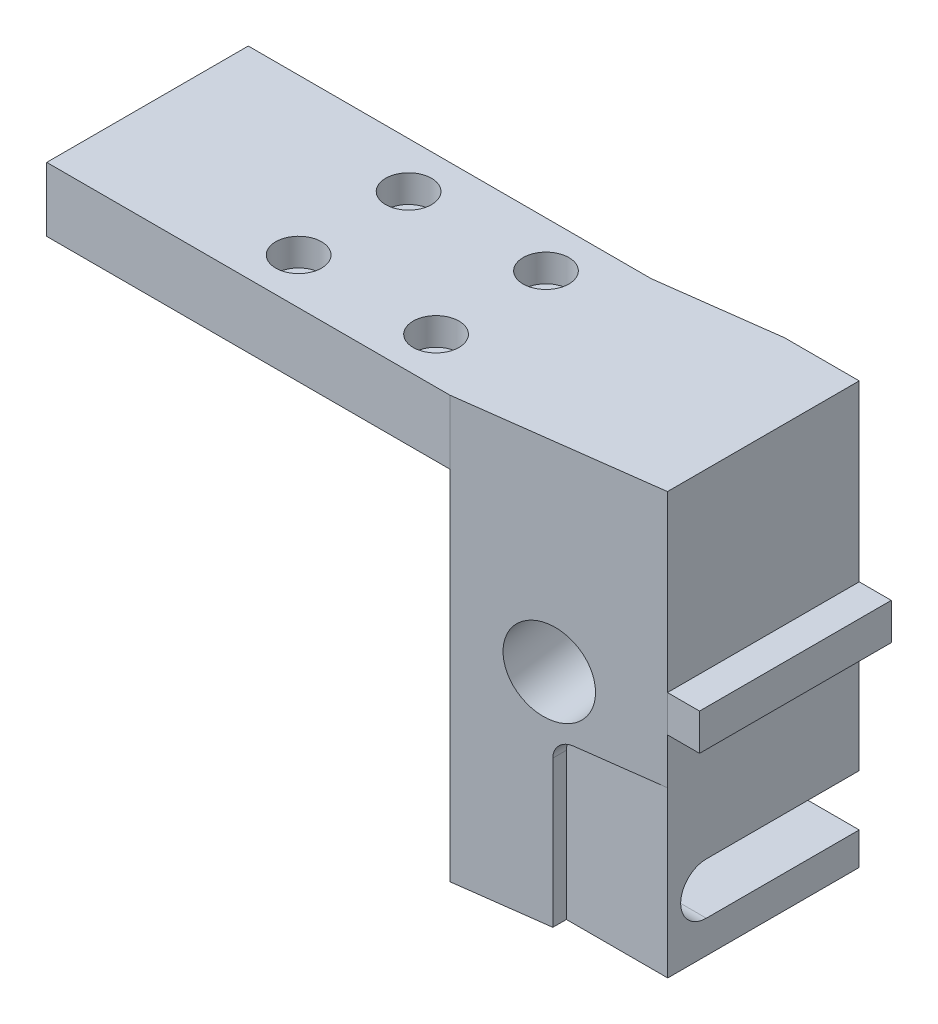
from build123d import *

# Parameters (mm, degrees)
EXTRUDE_1_DEPTH     = 23.69
CUT_EXTRUDE_1_REACH = 50.333
SKETCH_2_W          = 44
SKETCH_2_H          = 39
CUT_EXTRUDE_2_REACH = 75.348
CUT_EXTRUDE_3_DEPTH = 63.115721705
CUT_EXTRUDE_4_DEPTH = 2.79
CUT_EXTRUDE_5_REACH = 53.075
SKETCH_7_R          = 4.5
SKETCH_8_R          = 1.25
CUT_EXTRUDE_6_DEPTH = 8.5
SKETCH_10_R         = 1.45
CUT_EXTRUDE_7_DEPTH = 63.115721705
SKETCH_11_R         = 2.5
CUT_EXTRUDE_8_DEPTH = 3
SKETCH_12_R         = 2.25
CUT_EXTRUDE_9_DEPTH = 6


with BuildPart() as part:
    # 草图1 → 凸台-拉伸1 (new body)
    with BuildSketch(Plane.XY):
        Polygon((30.632183908, 5.365900383), (34.132183908, 5.365900383), (34.132183908, 1.365900383), (30.632183908, 1.365900383), (30.632183908, -21.634099617), (-34.367816092, -21.634099617), (-34.367816092, 24.365900383), (30.632183908, 24.365900383), align=None)
    extrude(amount=EXTRUDE_1_DEPTH)

    # 草图2 → 切除-拉伸1 (cut, up to next)
    with BuildSketch(Plane(origin=(0, 0, 0), x_dir=(-1, 0, 0), z_dir=(0, 0, -1)), mode=Mode.PRIVATE) as cut_extrude_1_sk1:
        with Locations((12.367816092, -2.134099617)):
            Rectangle(SKETCH_2_W, SKETCH_2_H)
    cut_extrude_1_tool1 = extrude(cut_extrude_1_sk1.sketch, amount=-CUT_EXTRUDE_1_REACH, mode=Mode.PRIVATE) & part.part
    add(cut_extrude_1_tool1.solids().sort_by_distance((-12.367816, -2.1341, 0))[0], mode=Mode.SUBTRACT)

    # 草图3 → 切除-拉伸2 (cut, up to next)
    with BuildSketch(Plane(origin=(30.632183908, 0, 0), x_dir=(0, 0, -1), z_dir=(1, 0, 0)), mode=Mode.PRIVATE) as cut_extrude_2_sk1:
        with BuildLine():
            Line((0, -18.084546462), (0, -12.484546462))
            Line((0, -12.484546462), (-16.69, -12.484546462))
            ThreePointArc((-16.69, -12.484546462), (-19.49, -15.284546462), (-16.69, -18.084546462))
            Line((-16.69, -18.084546462), (0, -18.084546462))
        make_face()
    cut_extrude_2_tool1 = extrude(cut_extrude_2_sk1.sketch, amount=-CUT_EXTRUDE_2_REACH, mode=Mode.PRIVATE) & part.part
    add(cut_extrude_2_tool1.solids().sort_by_distance((30.632184, -15.284546, 9.454896))[0], mode=Mode.SUBTRACT)

    # 草图4 → 切除-拉伸3 (cut, through all)
    with BuildSketch(Plane(origin=(0, 24.365900383, 0), x_dir=(1, 0, 0), z_dir=(0, 1, 0))):
        Polygon((9.632183908, -23.69), (34.132183908, -23.69), (34.132183908, -20.93), (30.632183908, -20.93), align=None)
        Polygon((-34.367816092, -1.69), (-34.367816092, 0), (22.482183908, 0), (9.632183908, -1.69), align=None)
    extrude(amount=-CUT_EXTRUDE_3_DEPTH, mode=Mode.SUBTRACT)

    # 草图5 → 切除-拉伸4 (cut)
    with BuildSketch(Plane.XY.offset(23.69)):
        with BuildLine():
            Line((30.632183908, -21.634099617), (19.572183908, -21.634099617))
            Line((19.572183908, -21.634099617), (19.572183908, -5.634099617))
            ThreePointArc((19.572183908, -5.634099617), (20.157970346, -4.219886054), (21.572183908, -3.634099617))
            Line((21.572183908, -3.634099617), (30.632183908, -3.634099617))
            Line((30.632183908, -3.634099617), (30.632183908, -21.634099617))
        make_face()
    extrude(amount=-CUT_EXTRUDE_4_DEPTH, mode=Mode.SUBTRACT)

    # 切除-拉伸5: up to this plane
    cut_extrude_5_end = Plane(origin=(22.482183908, -21.634099617, 0), z_dir=(0.13039463587890723, 0, 0.9914621722153636))
    # 草图7 → 切除-拉伸5 (cut, up to the surface)
    with BuildSketch(Plane(origin=(3.224230445, 0, 24.532188169), x_dir=(0.9914735684520677, 0, -0.1303079547108432), z_dir=(0.1303079547108432, 0, 0.9914735684520678)), mode=Mode.PRIVATE) as cut_extrude_5_sk1:
        with Locations((16.143060304, 2.365900383)):
            Circle(SKETCH_7_R)
    cut_extrude_5_tool1 = split(extrude(cut_extrude_5_sk1.sketch, amount=-CUT_EXTRUDE_5_REACH, mode=Mode.PRIVATE), bisect_by=cut_extrude_5_end, keep=Keep.BOTH, mode=Mode.PRIVATE)
    add(cut_extrude_5_tool1.solids().sort_by_distance((19.229648, 2.3659, 22.428619))[0], mode=Mode.SUBTRACT)

    # 草图8 → 切除-拉伸6 (cut)
    with BuildSketch(Plane.ZY.offset(34.367816092)):
        with Locations((7.69, 20.865900383)):
            Circle(SKETCH_8_R)
        with Locations((17.69, 20.865900383)):
            Circle(SKETCH_8_R)
    extrude(amount=-CUT_EXTRUDE_6_DEPTH, mode=Mode.SUBTRACT)

    # 草图10 → 切除-拉伸7 (cut, through all)
    with BuildSketch(Plane(origin=(0, 24.365900383, 0), x_dir=(1, 0, 0), z_dir=(0, 1, 0))):
        with Locations(Location((-11.867816092, -18.69, 0), (0, 0, 180))):
            Circle(SKETCH_10_R)
        with Locations(Location((-11.867816092, -6.69, 0), (0, 0, 180))):
            Circle(SKETCH_10_R)
        with Locations(Location((3.132183908, -18.69, 0), (0, 0, 180))):
            Circle(SKETCH_10_R)
        with Locations(Location((3.132183908, -6.69, 0), (0, 0, 180))):
            Circle(SKETCH_10_R)
    extrude(amount=-CUT_EXTRUDE_7_DEPTH, mode=Mode.SUBTRACT)

    # 草图11 → 切除-拉伸8 (cut)
    with BuildSketch(Plane(origin=(0, 24.365900383, 0), x_dir=(1, 0, 0), z_dir=(0, 1, 0))):
        with Locations(Location((-11.867816092, -6.69, 0), (0, 0, 180))):
            Circle(SKETCH_11_R)
        with Locations(Location((-11.867816092, -18.69, 0), (0, 0, 180))):
            Circle(SKETCH_11_R)
        with Locations(Location((3.132183908, -6.69, 0), (0, 0, 180))):
            Circle(SKETCH_11_R)
        with Locations(Location((3.132183908, -18.69, 0), (0, 0, 180))):
            Circle(SKETCH_11_R)
    extrude(amount=-CUT_EXTRUDE_8_DEPTH, mode=Mode.SUBTRACT)

    # 草图12 → 切除-拉伸9 (cut)
    with BuildSketch(Plane(origin=(0, 0, 0), x_dir=(-1, 0, 0), z_dir=(0, 0, -1))):
        with Locations((-26.632183908, 20.115900383)):
            Circle(SKETCH_12_R)
    extrude(amount=-CUT_EXTRUDE_9_DEPTH, mode=Mode.SUBTRACT)


solid = part.part
